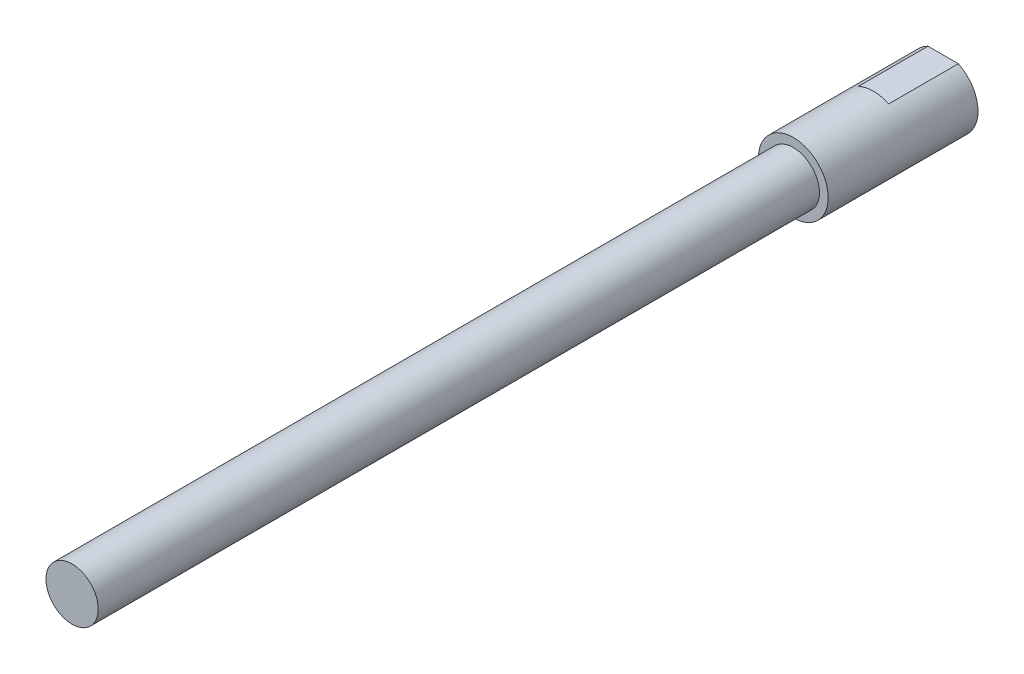
from build123d import *

# Parameters (mm, degrees)
SKETCH_1_R                   = 7.5
EXTRUDE_1_DEPTH              = 207
SKETCH_2_R                   = 10
EXTRUDE_2_DEPTH              = 43
SKETCH_3_OUTSIDE_W           = 72.318
SKETCH_3_OUTSIDE_H           = 72.318
SKETCH_3_OUTSIDE_W_2         = 23
SKETCH_3_OUTSIDE_H_2         = 18
CUT_EXTRUDE_1_DEPTH          = 20
HOLE_WIZARD_M8_1_D           = 6.8
HOLE_WIZARD_M8_1_DEPTH       = 18.25
HOLE_WIZARD_M8_1_CSINK_D     = 8.05
HOLE_WIZARD_M8_1_CSINK_ANGLE = 90
HOLE_WIZARD_M8_1_TIP         = 2.042926105


with BuildPart() as part:
    # 草图1 → 凸台-拉伸1 (new body)
    with BuildSketch(Plane.XY):
        Circle(SKETCH_1_R)
    extrude(amount=EXTRUDE_1_DEPTH)

    # 草图2 → 凸台-拉伸2 (add)
    with BuildSketch(Plane(origin=(0, 0, 0), x_dir=(-1, 0, 0), z_dir=(0, 0, -1))):
        Circle(SKETCH_2_R)
    extrude(amount=EXTRUDE_2_DEPTH)

    # 草图3 outside → 切除-拉伸1 (cut)
    with BuildSketch(Plane(origin=(0, 0, -43), x_dir=(-1, 0, 0), z_dir=(0, 0, -1))):
        Rectangle(SKETCH_3_OUTSIDE_W, SKETCH_3_OUTSIDE_H)
        Rectangle(SKETCH_3_OUTSIDE_W_2, SKETCH_3_OUTSIDE_H_2, mode=Mode.SUBTRACT)
    extrude(amount=-CUT_EXTRUDE_1_DEPTH, mode=Mode.SUBTRACT)

    # M8 螺纹孔1
    with Locations(Plane(origin=(0, 0, -43), x_dir=(-1, 0, 0), z_dir=(0, 0, -1))):
        with Locations((0, 0)):
            CounterSinkHole(HOLE_WIZARD_M8_1_D / 2, HOLE_WIZARD_M8_1_CSINK_D / 2, depth=HOLE_WIZARD_M8_1_DEPTH, counter_sink_angle=HOLE_WIZARD_M8_1_CSINK_ANGLE)
            with Locations((0, 0, -(HOLE_WIZARD_M8_1_DEPTH + HOLE_WIZARD_M8_1_TIP / 2))):  # 118° drill point
                Cone(0, HOLE_WIZARD_M8_1_D / 2, HOLE_WIZARD_M8_1_TIP, mode=Mode.SUBTRACT)


solid = part.part
